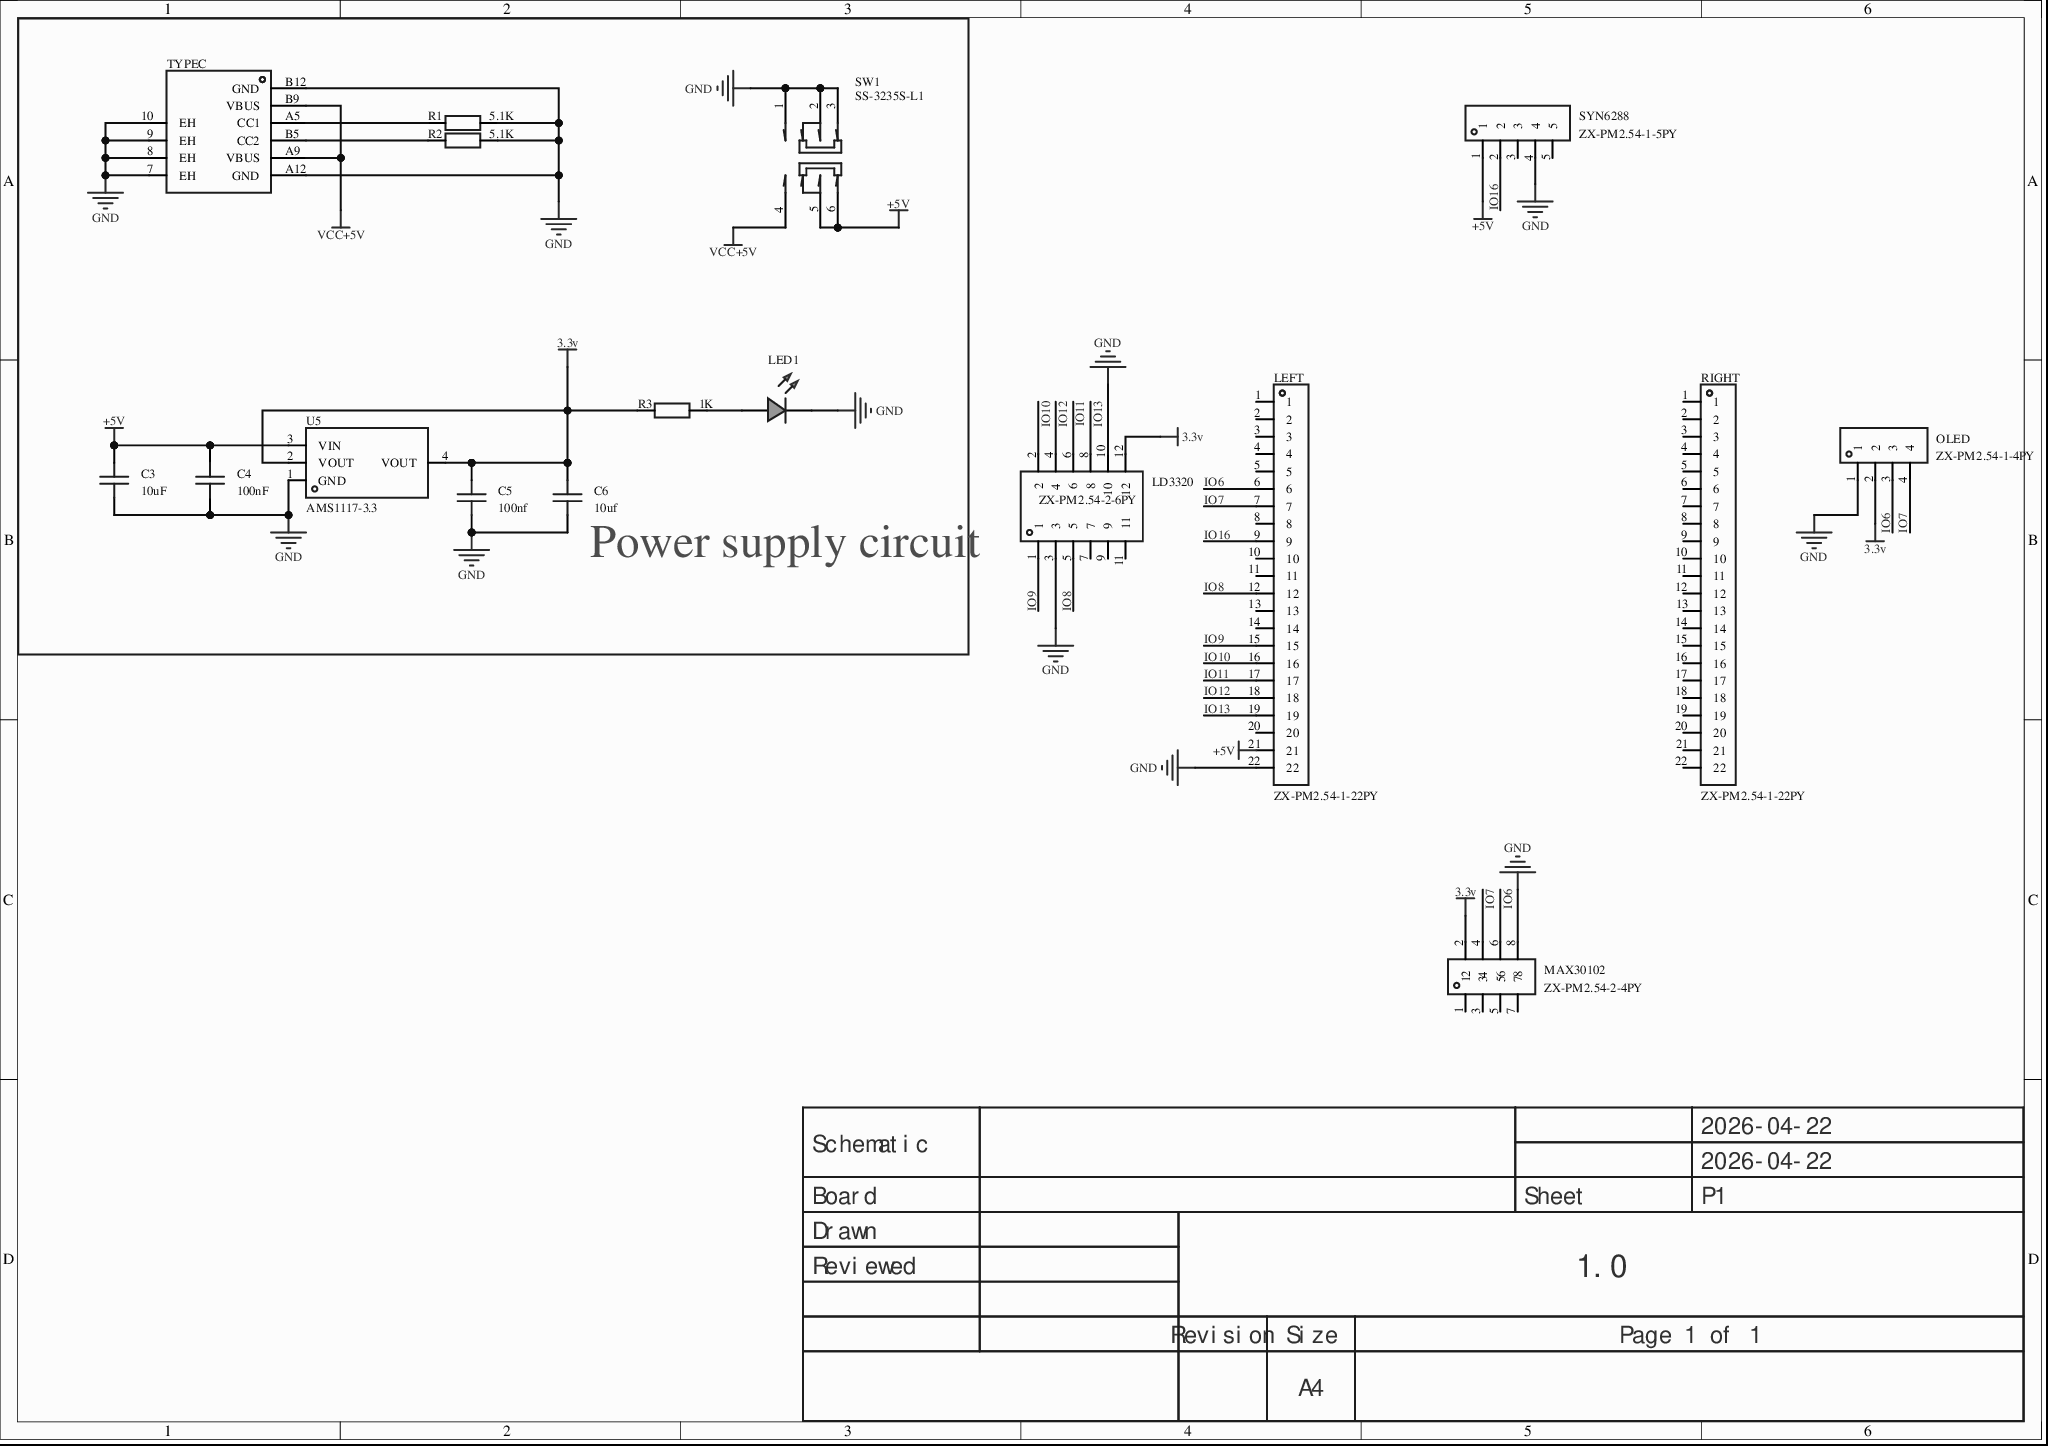
[diagram p0: MISC49905-3.schdoc]
# Altium project MISC49905-2.PrjPcb
1 sheet, 17 parts. Net scope: global (net labels, ports and power ports of the same name join across sheets).
Board file: MISC49905.pcbdoc

## Sheet MISC49905-3.schdoc
size 297 x 209 mm; Version: V1.0; @Project Name: MISC49905; @Update Date: 2026-04-22; @Create Date: 2026-04-22; @Board Name: MISC49905; @Create Time: 16:58:48; @Page Count: 1; @Page No: 1; @Schematic Name: MISC49905; @Update Time: 16:58:48; Size: A4

### Parts
C3  10uF  [C0603]
C4  100nF  [C0603]
C5  100nf  [C0603]
C6  10uf  [C0603]
LD3320  ZX-PM2.54-2-6PY  [HDR-TH_12P-P2.54-V-F-R2-C6-S2.54]
LED1  (no value)  [LED_0805]
LEFT  ZX-PM2.54-1-22PY  [HDR-TH_22P-P2.54-V-F]
MAX30102  ZX-PM2.54-2-4PY  [HDR-TH_8P-P2.54-V-F-R2-C4-S2.54]
OLED  ZX-PM2.54-1-4PY  [HDR-TH_4P-P2.54-V-F]
R1  5.1K  [R0603]
R2  5.1K  [R0603]
R3  1K  [R0603]
RIGHT  ZX-PM2.54-1-22PY  [HDR-TH_22P-P2.54-V-F]
SW1  SS-3235S-L1  [SW-SMD_SS-3235S-LX]
SYN6288  ZX-PM2.54-1-5PY  [HDR-TH_5P-P2.54-V-F-B]
TYPEC  (no value)  [USB_ TYPE-C-6P]
U5  AMS1117-3.3  [SOT-223-3_L6.5-W3.4-P2.30-LS7.0-BR]

### Blocks framed on the sheet
Power supply circuit: C3-C6 LED1 R1-R3 SW1 TYPEC U5

### Nets
3.3v: C5.2 C6.2 LD3320.12 MAX30102.2 OLED.2 R3.1 U5.2(VOUT) U5.4(VOUT)
+5V: C3.2 C4.2 LEFT.21 SW1.5 SW1.6 SYN6288.1 U5.3(VIN)
GND: C3.1 C4.1 C5.1 C6.1 LD3320.3 LD3320.10 LED1.1(C) LEFT.22 MAX30102.8 OLED.1 R1.2 R2.2 SW1.1 SW1.2 SW1.3 SYN6288.4 TYPEC.7(EH) TYPEC.8(EH) TYPEC.9(EH) TYPEC.10(EH) TYPEC.A12(GND) TYPEC.B12(GND) U5.1(GND)
VCC+5V: SW1.4 TYPEC.A9(VBUS) TYPEC.B9(VBUS)
IO6: LEFT.6 MAX30102.6 OLED.3
IO7: LEFT.7 MAX30102.4 OLED.4
IO8: LD3320.5 LEFT.12
IO9: LD3320.1 LEFT.15
IO10: LD3320.2 LEFT.16
IO11: LD3320.6 LEFT.17
IO12: LD3320.4 LEFT.18
IO13: LD3320.8 LEFT.19
IO16: LEFT.9 SYN6288.2
NetLED1_2: LED1.2(A) R3.2
NetR1_1: R1.1 TYPEC.A5(CC1)
NetR2_1: R2.1 TYPEC.B5(CC2)

Not connected (* = marked no-connect by the designer): LD3320 7* 9* 11*; LEFT 1* 2* 3* 4* 5* 8* 10* 11* 13* 14* 20*; MAX30102 1* 3* 5* 7*; RIGHT 1* 2* 3* 4* 5* 6* 7* 8* 9* 10* 11* 12* 13* 14* 15* 16* 17* 18* 19* 20* 21* 22*; SYN6288 3* 5*

### Notes on the sheet
- 2026-04-22
- Schematic
- Board
- Sheet
- P1
- Drawn
- Reviewed
- 1.0
- Revision
- Size
- A4
- Page 1 of 1

### Library data of the parts
C3 C5 = CL10A106MA8NRNC: Capacitance: 10uF; tolerance: ±20%; rated voltage: 25V; temperature coefficient: X5R;; Manufacturer: SAMSUNG(三星); Add into BOM: yes; 3D Model: ac125912035d415993ca9572d50418b1; 3D Model Transform: 62.992,31.496,0,0,0,0,0,0,0; ModelName: C0603_L1.6-W0.8-H0.8; Symbol: CL10A106MA8NRNC; Device: CL10A106MA8NRNC; Convert to PCB: yes; Supplier Footprint: 0603; LCSC Part Name: 10uF ±20% 25V; Manufacturer Part: CL10A106MA8NRNC; JLCPCB Part Class: Basic Part; Datasheet: https://example.com/datasheet/CL10A106MA8NRNC/97651.html; Supplier: LCSC; Tolerance: ±20%; Voltage Rating: 25V; Temperature Coefficient: X5R; FootprintName: C0603
  C3: Value: 10uF; Supplier Part: C96446
  C5: Value: 100nf
C4 C6 = CAP_0603: Symbol: Capacitance; 3D Model: ac125912035d415993ca9572d50418b10819f05c4eef4c71ace90d822a990e87; 3D Model Transform: 62.992,31.496,0,0,0,0,0,0,0; ConvertToPcb: yes; ModelName: C0603_L1.6-W0.8-H0.8; Device: CAP_0603; Supplier Footprint: 0603; AddInBom: yes; FootprintName: C0603
  C4: Value: 100nF
  C6: Value: 10uf
LD3320 = ZX-PM2.54-2-6PY: Socket structure: 2x6P; pitch: 2.54mm; row spacing: 2.54mm; round/square hole: square; mounting: through-hole; rows: double row; total positions: 12P; rated current: 3A; rated voltage: -; hole direction: top; plastic height: 8.5mm; contact material: brass; contact plating: gold; working temperature: -40℃~+105℃;; Manufacturer: Megastar(兆星); Add into BOM: yes; 3D Model: 95d1f1a5666d46438f9c767a173340ed; 3D Model Transform: 615.7468,196.85,0,0,0,0,0,0,-129.921; PIN Length: 3.2mm; ModelName: HDR-TH_12P-P2.54-F-LI-2X6P; Symbol: ZX-PM2.54-2-6PY; Device: ZX-PM2.54-2-6PY; Convert to PCB: yes; LCSC Part Name: 2x6P 间距:2.54mm 直插; Supplier Part: C7499342; Manufacturer Part: ZX-PM2.54-2-6PY; Supplier Footprint: 插件,P=2.54mm; JLCPCB Part Class: Extended Part; Datasheet: https://example.com/datasheet/ZX-PM2.54-2-6PY/8574003.html; Supplier: LCSC; Holes Structure: 2x6P; Pitch: 2.54mm; Row Spacing: 2.54mm; Circular Hole / Square Hole: Square hole; Mounting Type: Through-hole; Number of Rows: Double row; Number of Positions: 12P; Current Rating: 3A; Voltage Rating (Max): -; Holes Direction: Top; Insulation Height: 8.5mm; Contact Material: Brass; Contact Plating: Gold; Operating Temperature: -40℃~+105℃; FootprintName: HDR-TH_12P-P2.54-V-F-R2-C6-S2.54
LED1 = LED_0805-G: Symbol: LED_G; Convert to PCB: yes; 3D Model: 381ae4d721d6485eaad9d0ca067812b50819f05c4eef4c71ace90d822a990e87; 3D Model Transform: 63.9,39.8,31.9,0,0,0,0,0,0; ModelName: LED-0805_G; Device: LED_0805-G; Add into BOM: yes; Supplier Footprint: 0805; FootprintName: LED_0805
LEFT RIGHT = ZX-PM2.54-1-22PY: Socket structure: 1x22P; pitch: 2.54mm; row spacing: -; round/square hole: square; mounting: through-hole; rows: single row; total positions: 22P; rated current: 3A; rated voltage: -; hole direction: top; plastic height: 8.5mm; contact material: brass; contact plating: gold; working temperature: -40℃~+105℃;; Manufacturer: Megastar(兆星); Add into BOM: yes; 3D Model: 0181345c91514c0db21026e917058281; 3D Model Transform: 2199.99552,98.425,0,0,0,0,0,0,-125.984; PIN Length: 3.2mm; Symbol: ZX-PM2.54-1-22PY; Device: ZX-PM2.54-1-22PY; Convert to PCB: yes; LCSC Part Name: 1x22P 间距:2.54mm 直插; Supplier Part: C7499337; Manufacturer Part: ZX-PM2.54-1-22PY; Supplier Footprint: 插件,P=2.54mm; JLCPCB Part Class: Extended Part; Datasheet: https://example.com/datasheet/ZX-PM2.54-1-22PY/8573998.html; Supplier: LCSC; Holes Structure: 1x22P; Pitch: 2.54mm; Row Spacing: -; Circular Hole / Square Hole: Square hole; Mounting Type: Through-hole; Number of Rows: Single row; Number of Positions: 22P; Current Rating: 3A; Voltage Rating (Max): -; Holes Direction: Top; Insulation Height: 8.5mm; Contact Material: Brass; Contact Plating: Gold; Operating Temperature: -40℃~+105℃; FootprintName: HDR-TH_22P-P2.54-V-F; ModelName: HDR-TH_22P-P2.54-V-F
MAX30102 = ZX-PM2.54-2-4PY: Socket structure: 2x4P; pitch: 2.54mm; row spacing: 2.54mm; round/square hole: square; mounting: through-hole; rows: double row; total positions: 8P; rated current: 3A; rated voltage: -; hole direction: top; plastic height: 8.5mm; contact material: brass; contact plating: gold; working temperature: -40℃~+105℃;; Manufacturer: Megastar(兆星); Add into BOM: yes; 3D Model: 52f9c7b3691648c0a1959c61eae44590; 3D Model Transform: 415.7472,196.85,0,0,0,0,0,0,-118.11; PIN Length: 3.2mm; ModelName: HDR-TH_8P-P2.54-F-LI-2X4P; Symbol: ZX-PM2.54-2-4PY; Device: ZX-PM2.54-2-4PY; Convert to PCB: yes; LCSC Part Name: 2x4P 间距:2.54mm 直插; Supplier Part: C7499340; Manufacturer Part: ZX-PM2.54-2-4PY; Supplier Footprint: 插件,P=2.54mm; JLCPCB Part Class: Extended Part; Datasheet: https://example.com/datasheet/ZX-PM2.54-2-4PY/8574001.html; Supplier: LCSC; Holes Structure: 2x4P; Pitch: 2.54mm; Row Spacing: 2.54mm; Circular Hole / Square Hole: Square hole; Mounting Type: Through-hole; Number of Rows: Double row; Number of Positions: 8P; Current Rating: 3A; Voltage Rating (Max): -; Holes Direction: Top; Insulation Height: 8.5mm; Contact Material: Brass; Contact Plating: Gold; Operating Temperature: -40℃~+105℃; FootprintName: HDR-TH_8P-P2.54-V-F-R2-C4-S2.54
OLED = ZX-PM2.54-1-4PY: Socket structure: 1x4P; pitch: 2.54mm; row spacing: -; round/square hole: square; mounting: through-hole; rows: single row; total positions: 4P; rated current: 3A; rated voltage: -; hole direction: top; plastic height: 8.5mm; contact material: brass; contact plating: gold; working temperature: -40℃~+105℃;; Manufacturer: Megastar(兆星); Add into BOM: yes; 3D Model: d187812051054f85879fcaa51a310d8e; 3D Model Transform: 419.6842,98.464,0,0,0,0,0,0,-118.11; PIN Length: 3.2mm; Symbol: ZX-PM2.54-1-4PY; Device: ZX-PM2.54-1-4PY; Convert to PCB: yes; LCSC Part Name: 1x4P 间距:2.54mm 直插; Supplier Part: C7499324; Manufacturer Part: ZX-PM2.54-1-4PY; Supplier Footprint: 插件,P=2.54mm; JLCPCB Part Class: Extended Part; Datasheet: https://example.com/datasheet/ZX-PM2.54-1-4PY/8573985.html; Supplier: LCSC; Holes Structure: 1x4P; Pitch: 2.54mm; Row Spacing: -; Circular Hole / Square Hole: Square hole; Mounting Type: Through-hole; Number of Rows: Single row; Number of Positions: 4P; Current Rating: 3A; Voltage Rating (Max): -; Holes Direction: Top; Insulation Height: 8.5mm; Contact Material: Brass; Contact Plating: Gold; Operating Temperature: -40℃~+105℃; FootprintName: HDR-TH_4P-P2.54-V-F; ModelName: HDR-TH_4P-P2.54-V-F
R1-R3 = Res_0603: Symbol: Resistor; 3D Model: fc143cca1e79419f9cd78b61e9279f080819f05c4eef4c71ace90d822a990e87; 3D Model Transform: 31.8897,63.7794,0,90,0,0,0,0,0; ConvertToPcb: yes; Device: Res_0603; Supplier Footprint: 0603; AddInBom: yes; FootprintName: R0603; ModelName: R0603
  R1 R2: Value: 5.1K
  R3: Value: 1K
SW1 = SS-3235S-L1: Circuit structure: DPDT; mounting: horizontal SMD; switch color: black; rated current: 50mA; rated voltage: 12V; service life: 1万 cycles;; Manufacturer: XKB Connection(中国星坤); AddInBom: yes; ModelId: e98810a9d4c646b4962907642f59f8260819f05c4eef4c71ace90d822a990e87; ModelTransform: 356.299,271.653,0,0,0,0,0.002,-0.004,0; Actuator Style: Rectangular post; Switch Height: 3.2mm; Symbol: SS-3235S-L1; Device: SS-3235S-L1; LCSC Part Name: 柄长2mm 卧贴双档 滑动开关; SupplierPart: C500055; ManufacturerPart: SS-3235S-L1; Supplier Footprint: SMD,9.1x3.6mm; JLCPCB Part Class: Extended Part; Datasheet: https://example.com/datasheet/SS-3235S-L1/512181.html; Supplier: LCSC; ConvertToPcb: yes; FootprintName: SW-SMD_SS-3235S-LX; ModelName: SW-SMD_SS-3235S-LX; Circuit: DPDT; Termination Style: Gull wing; Length: 9.1mm; Width: 3.55mm; Mounting Type: Horizontal SMD; Actuator Color: Black; Current Rating: 50mA; Voltage Rating: 12V; Life: 1万 cycles; Operating Temperature: -40℃~+85℃
SYN6288 = ZX-PM2.54-1-5PY: Socket structure: 1x5P; pitch: 2.54mm; row spacing: -; round/square hole: square; mounting: through-hole; rows: single row; total positions: 5P; rated current: 3A; rated voltage: -; hole direction: top; plastic height: 8.5mm; contact material: brass; contact plating: gold; working temperature: -40℃~+105℃;; Manufacturer: Megastar(兆星); Add into BOM: yes; 3D Model: 71ad630020884b4a8e44edd825ca70bd; 3D Model Transform: 515.747,98.425,0,0,0,0,0,0,-125.984; PIN Length: 3.2mm; Symbol: ZX-PM2.54-1-5PY; Device: ZX-PM2.54-1-5PY; Convert to PCB: yes; LCSC Part Name: 1x5P 间距:2.54mm 直插; Supplier Part: C7499325; Manufacturer Part: ZX-PM2.54-1-5PY; Supplier Footprint: 插件,P=2.54mm; JLCPCB Part Class: Extended Part; Datasheet: https://example.com/datasheet/ZX-PM2.54-1-5PY/8573986.html; Supplier: LCSC; Holes Structure: 1x5P; Pitch: 2.54mm; Row Spacing: -; Circular Hole / Square Hole: Square hole; Mounting Type: Through-hole; Number of Rows: Single row; Number of Positions: 5P; Current Rating: 3A; Voltage Rating (Max): -; Holes Direction: Top; Insulation Height: 8.5mm; Contact Material: Brass; Contact Plating: Gold; Operating Temperature: -40℃~+105℃; FootprintName: HDR-TH_5P-P2.54-V-F-B; ModelName: HDR-TH_5P-P2.54-V-F-B
TYPEC = USB_ Type-C-6P: 3D Model: d4f492a4e6024845a13b3f6a4ef2d2cb0819f05c4eef4c71ace90d822a990e87; 3D Model Transform: 352.362,281.496,0,0,0,0,0,-47.244,-39.37; AddInBom: yes; ModelName: USB-SMD_U262-061N-4BVC11; Symbol: USB_ TYPE-C-6P; Device: USB_ Type-C-6P; Supplier Footprint: SMD; ConvertToPcb: yes; FootprintName: USB_ TYPE-C-6P
U5 = AMS1117-3.3_C6186: Output type: fixed; working voltage: 15V; output voltage: 3.3V; output current: 1A; ripple rejection (PSRR): 72dB@(120Hz); output polarity: positive;; Manufacturer: AMS; AddInBom: yes; ModelId: 925194bf9823436183a3e0b978a8d0760819f05c4eef4c71ace90d822a990e87; ModelName: SOT-223-4P_L6.5-W3.5-H1.6-LS7.0-P2.30; ModelTransform: 279.89794,255.905,0,180,0,0,-3.9385,-0.0005,0; Voltage Dropout: 1.1V@(800mA); standby current: 5mA; Noise: 0.003%Vout; Number of Outputs: 1; Symbol: AMS1117-3.3; Device: AMS1117-3.3_C6186; LCSC Part Name: 3.3V 1A 15V; SupplierPart: C6186; ManufacturerPart: AMS1117-3.3; Supplier Footprint: SOT-223; JLCPCB Part Class: Basic Part; Datasheet: https://example.com/datasheet/AMS1117-3.3/6652.html; Supplier: LCSC; ConvertToPcb: yes; FootprintName: SOT-223-3_L6.5-W3.4-P2.30-LS7.0-BR; Output Type: Fixed; Voltage - Supply: 15V; Output Voltage: 3.3V; Output Current: 1A; Power Supply Rejection Ratio (PSRR): 72dB@(120Hz); Features: Overcurrent protection; thermal shutdown; Operating Temperature: -40℃~+125℃; Output Configuration: Positive